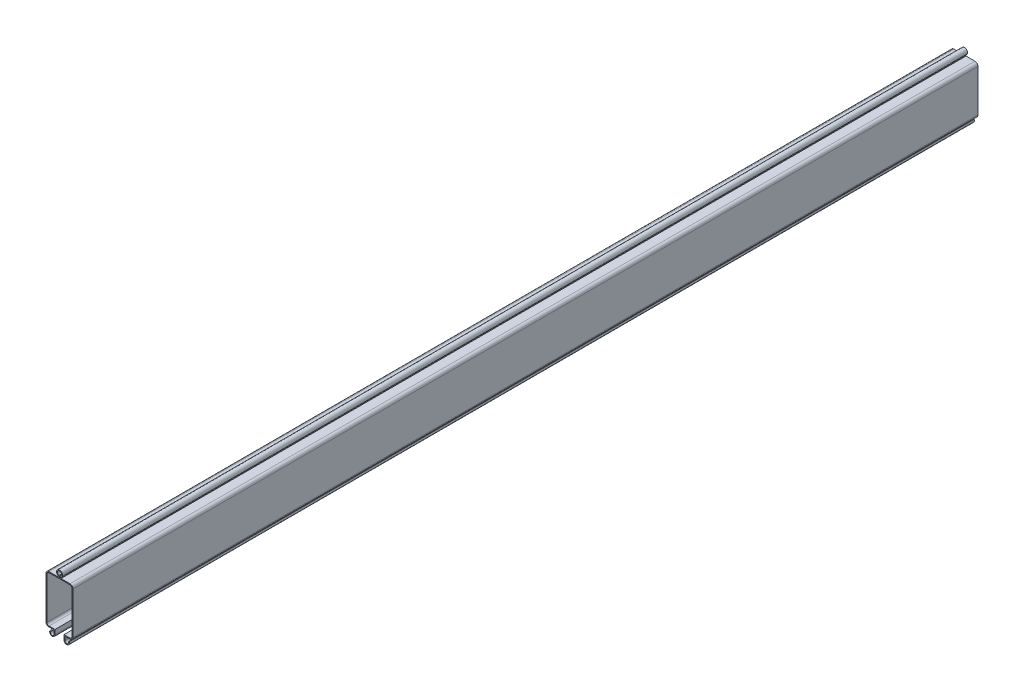
SolidWorks part; units mm, degrees
ref_plane "Front Plane" through (0, 0, 0) normal (0, 0, 1) x (1, 0, 0)
ref_plane "Top Plane" through (0, 0, 0) normal (0, 1, 0) x (1, 0, 0)
ref_plane "Right Plane" through (0, 0, 0) normal (1, 0, 0) x (0, 0, -1)
other "Configuration Table"
sketch "Sketch1" plane through (0, 0, 0) normal (0, 0, 1) x (1, 0, 0)
  line L0 (0, 80) -> (0, -114.6613) construction
  line L1 (-35, 80) -> (-5, 80)
  line L2 (-45, 70) -> (-45, -70)
  line L3 (-35, -80) -> (-18, -80)
  line L4 (45, 70) -> (45, -70)
  line L5 (-45, 80) -> (45, -80) construction
  line L6 (-45, -80) -> (45, 80) construction
  line L7 (-18, -92.3951) -> (-18, -80)
  line L8 (-5, 83.72) -> (-5, 80)
  line L9 (18, -80) -> (35, -80)
  line L10 (5, 83.72) -> (5, 80)
  line L11 (5, 80) -> (35, 80)
  line L12 (18, -92.3951) -> (18, -80)
  line L13 (15, -92.3951) -> (15, -77)
  line L14 (15, -77) -> (35, -77)
  line L15 (42, 70) -> (42, -70)
  line L16 (2, 77) -> (35, 77)
  line L17 (2, 85.672) -> (2, 77)
  line L18 (-2, 85.672) -> (-2, 77)
  line L19 (-35, 77) -> (-2, 77)
  line L20 (-42, 70) -> (-42, -70)
  line L21 (-35, -77) -> (-15, -77)
  line L22 (-15, -92.3951) -> (-15, -77)
  line L23 (-29.5037, -90.0943) -> (-32.2729, -88.9405)
  line L24 (32.2729, -88.9405) -> (29.5037, -90.0943)
  arc A0 (-29.5037, -90.0943) -> (-18, -92.3951) centre (-23.9819, -92.3951) ccw
  arc A1 (5, 83.72) -> (-5, 83.72) centre (0, 92.3802) ccw
  arc A2 (-45, -70) -> (-35, -80) centre (-35, -70) ccw
  arc A3 (29.5037, -90.0943) -> (18, -92.3951) centre (23.9819, -92.3951) cw
  arc A4 (35, -80) -> (45, -70) centre (35, -70) ccw
  arc A5 (35, 80) -> (45, 70) centre (35, 70) cw
  arc A6 (-35, 80) -> (-45, 70) centre (-35, 70) ccw
  arc A7 (32.2729, -88.9405) -> (15, -92.3951) centre (23.9819, -92.3951) cw
  arc A8 (35, -77) -> (42, -70) centre (35, -70) ccw
  arc A9 (35, 77) -> (42, 70) centre (35, 70) cw
  arc A10 (2, 85.672) -> (-2, 85.672) centre (0, 92.3802) ccw
  arc A11 (-35, 77) -> (-42, 70) centre (-35, 70) ccw
  arc A12 (-42, -70) -> (-35, -77) centre (-35, -70) ccw
  arc A13 (-32.2729, -88.9405) -> (-15, -92.3951) centre (-23.9819, -92.3951) ccw
  point P0 (0, 0)
  dimension "D3" = 20
  dimension "D6" = 10
  dimension "D1" = 90
  dimension "D2" = 160
  dimension "D4" = 10
  dimension "D5" = 5
  dimension "D8" = 30
  dimension "D7" = 3
extrude "Boss-Extrude1" add sketch "Sketch1" along normal blind 3017
